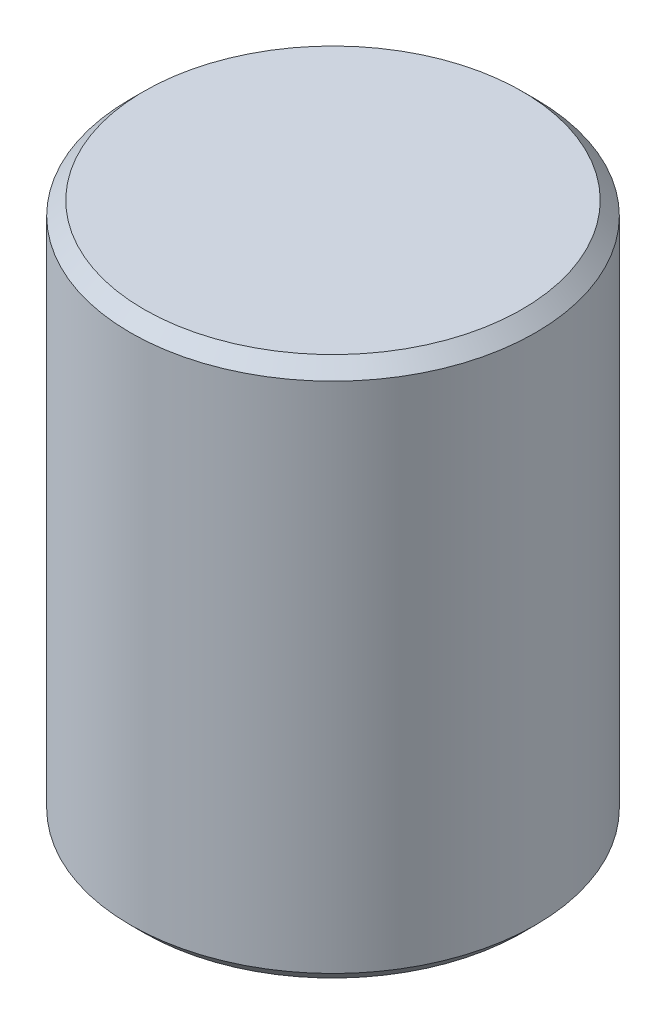
from build123d import *

# Parameters (mm, degrees)
SKETCH1_R           = 3
BOSS_EXTRUDE1_DEPTH = 8
CHAMFER1_SIZE       = 0.2


with BuildPart() as part:
    # Sketch1 → Boss-Extrude1 (new body)
    with BuildSketch(Plane(origin=(0, 0, 0), x_dir=(1, 0, 0), z_dir=(0, 1, 0))):
        with Locations(Location((0, 0, 0), (0, 0, 270))):
            Circle(SKETCH1_R)
    extrude(amount=BOSS_EXTRUDE1_DEPTH)

    # Chamfer1
    chamfer1_edges = [part.edges().sort_by_distance(p)[0] for p in [
        (0, 0, -3),
        (0, 8, -3),
    ]]
    chamfer(chamfer1_edges, length=CHAMFER1_SIZE)


solid = part.part
